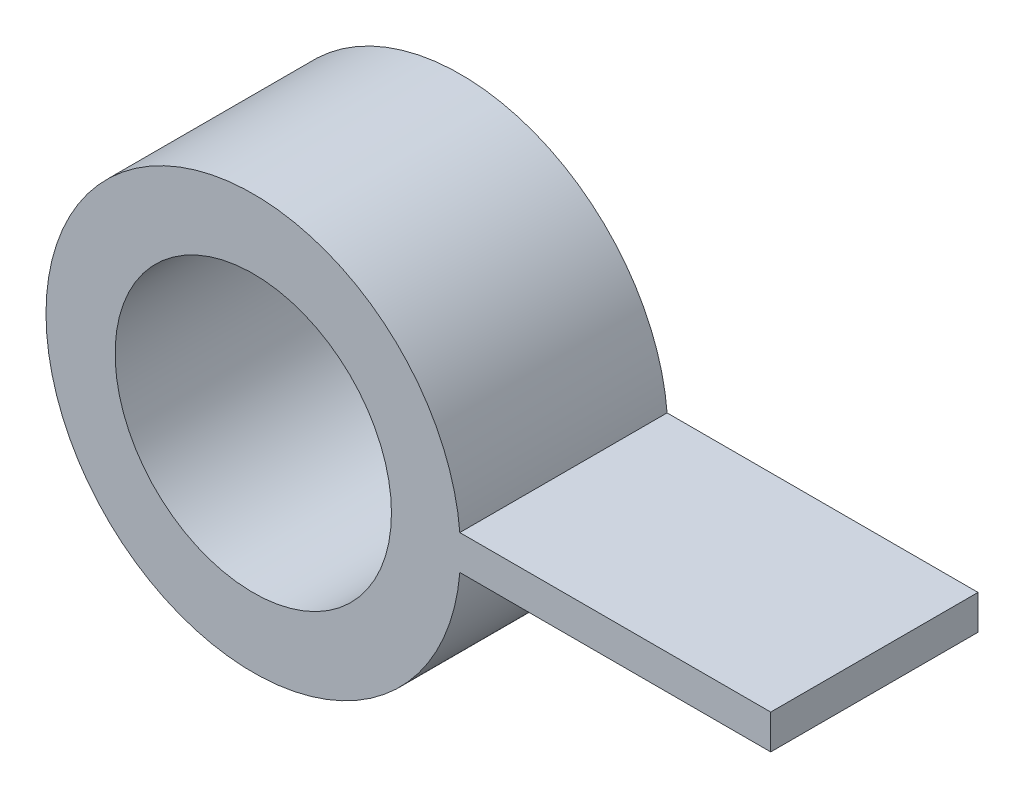
SolidWorks part; units mm, degrees
ref_plane "前视基准面" through (0, 0, 0) normal (0, 0, 1) x (1, 0, 0)
ref_plane "上视基准面" through (0, 0, 0) normal (0, 1, 0) x (1, 0, 0)
ref_plane "右视基准面" through (0, 0, 0) normal (1, 0, 0) x (0, 0, -1)
sketch "草图1" plane through (0, 0, 0) normal (0, 0, 1) x (1, 0, 0)
  circle A0 centre (0, 0) radius 8
  circle A1 centre (0, 0) radius 12
  dimension "D1" = 16
  dimension "D2" = 24
extrude "凸台-拉伸1" add sketch "草图1" along normal mid plane 12
sketch "草图2" plane through (0, 0, 6) normal (0, 0, 1) x (1, 0, 0)
  line L0 (11.9583, 1) -> (29.9583, 1)
  line L1 (29.9583, 1) -> (29.9583, -1)
  line L2 (29.9583, -1) -> (11.9583, -1)
  line L3 (11.9583, -1) -> (11.9583, 1)
  circle A0 centre (0, 0) radius 12 construction
  dimension "D1" = 2
  dimension "D2" = 18
extrude "凸台-拉伸2" add sketch "草图2" against normal up to surface (12 mm away) up to face at (12, 0, -6)
